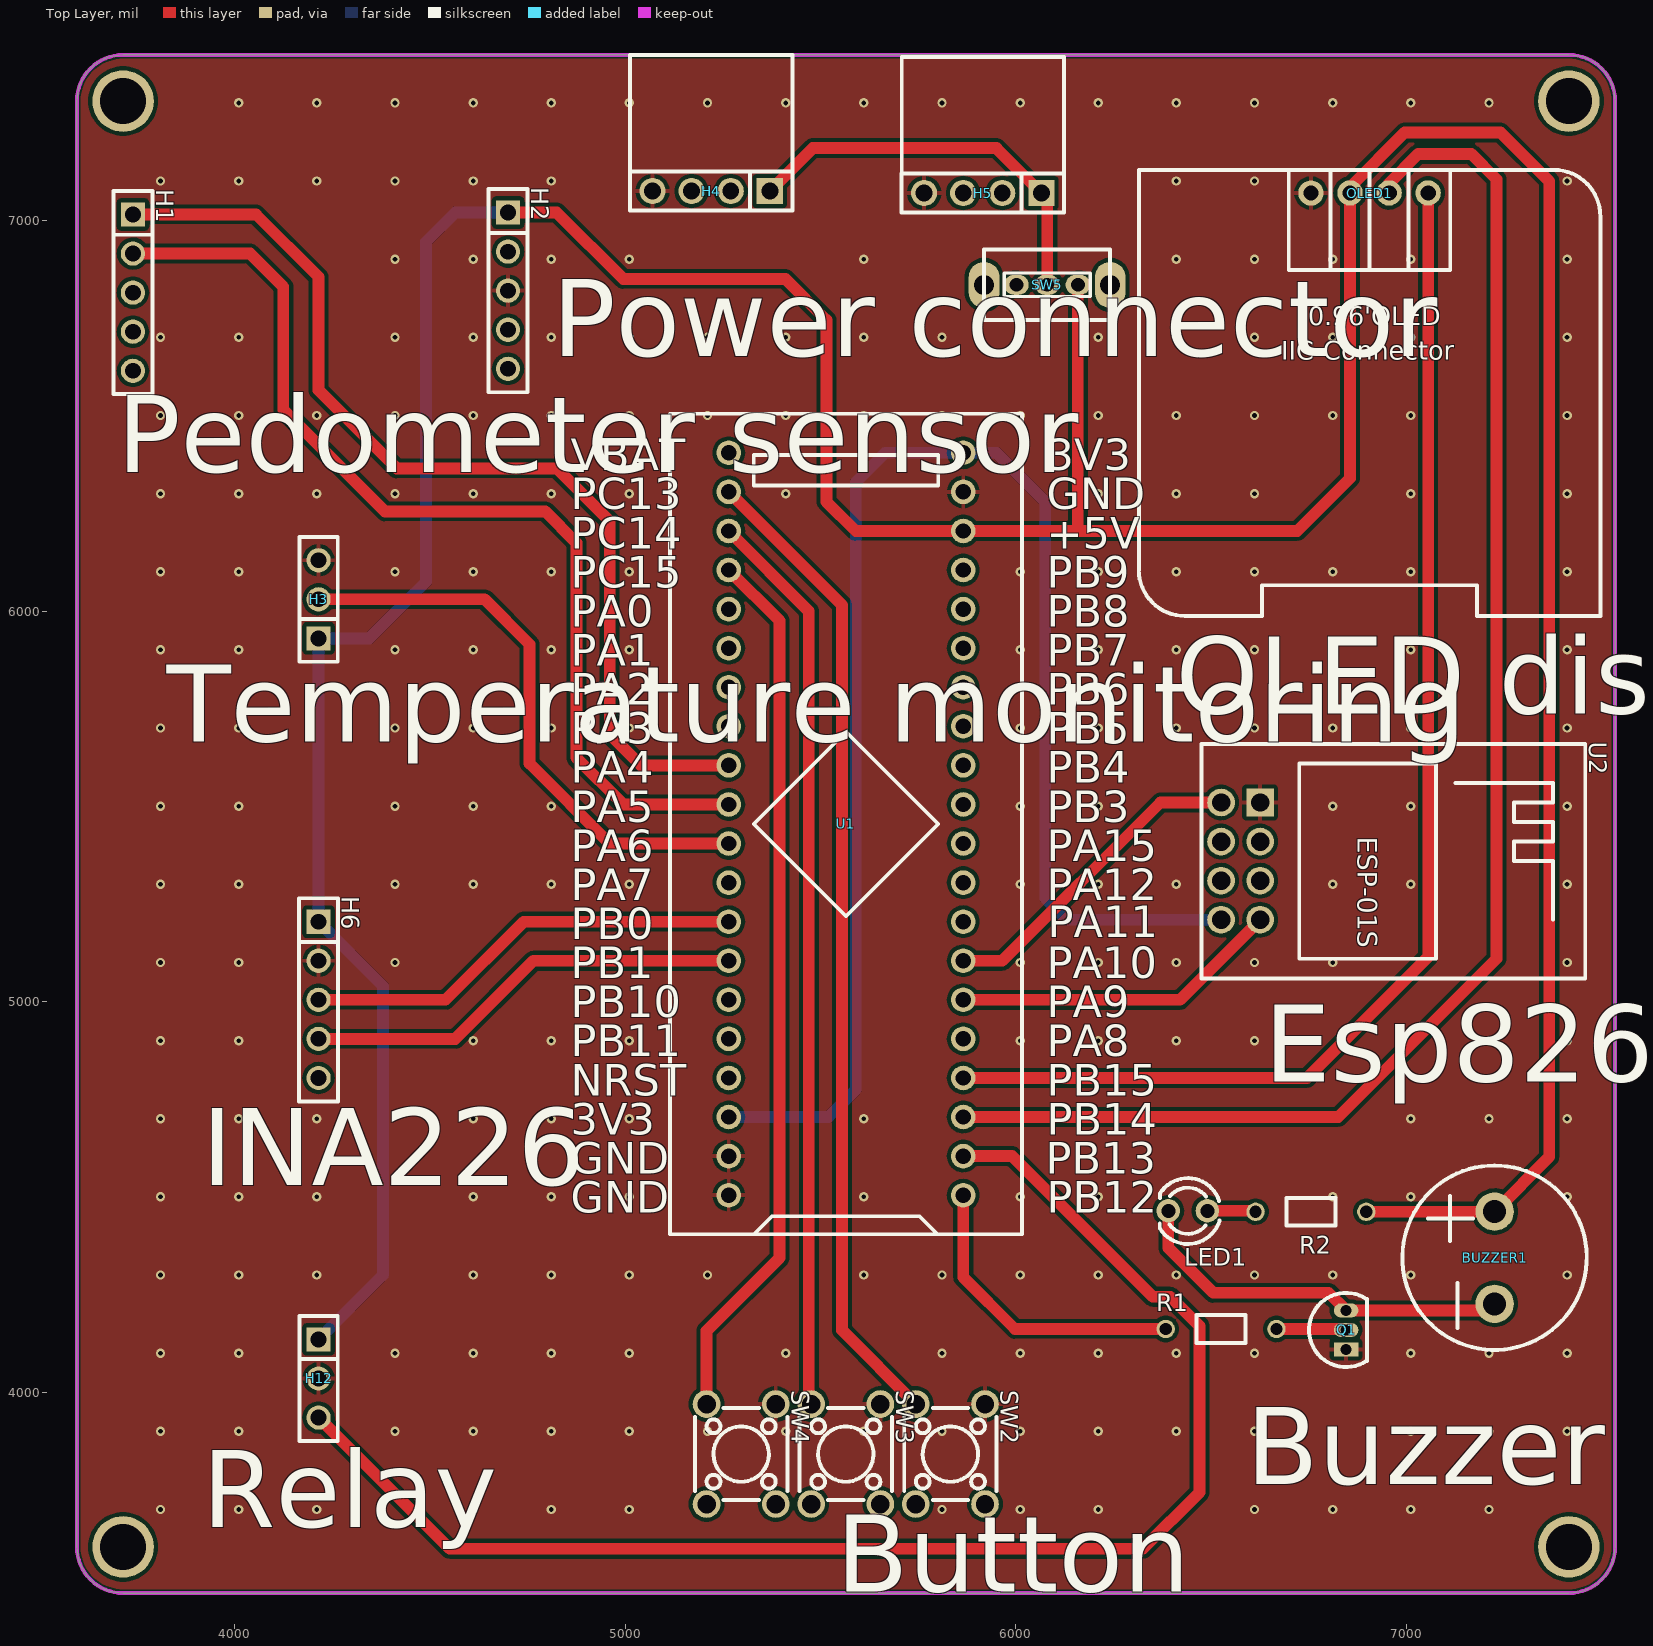
[diagram p0: Top Layer view]
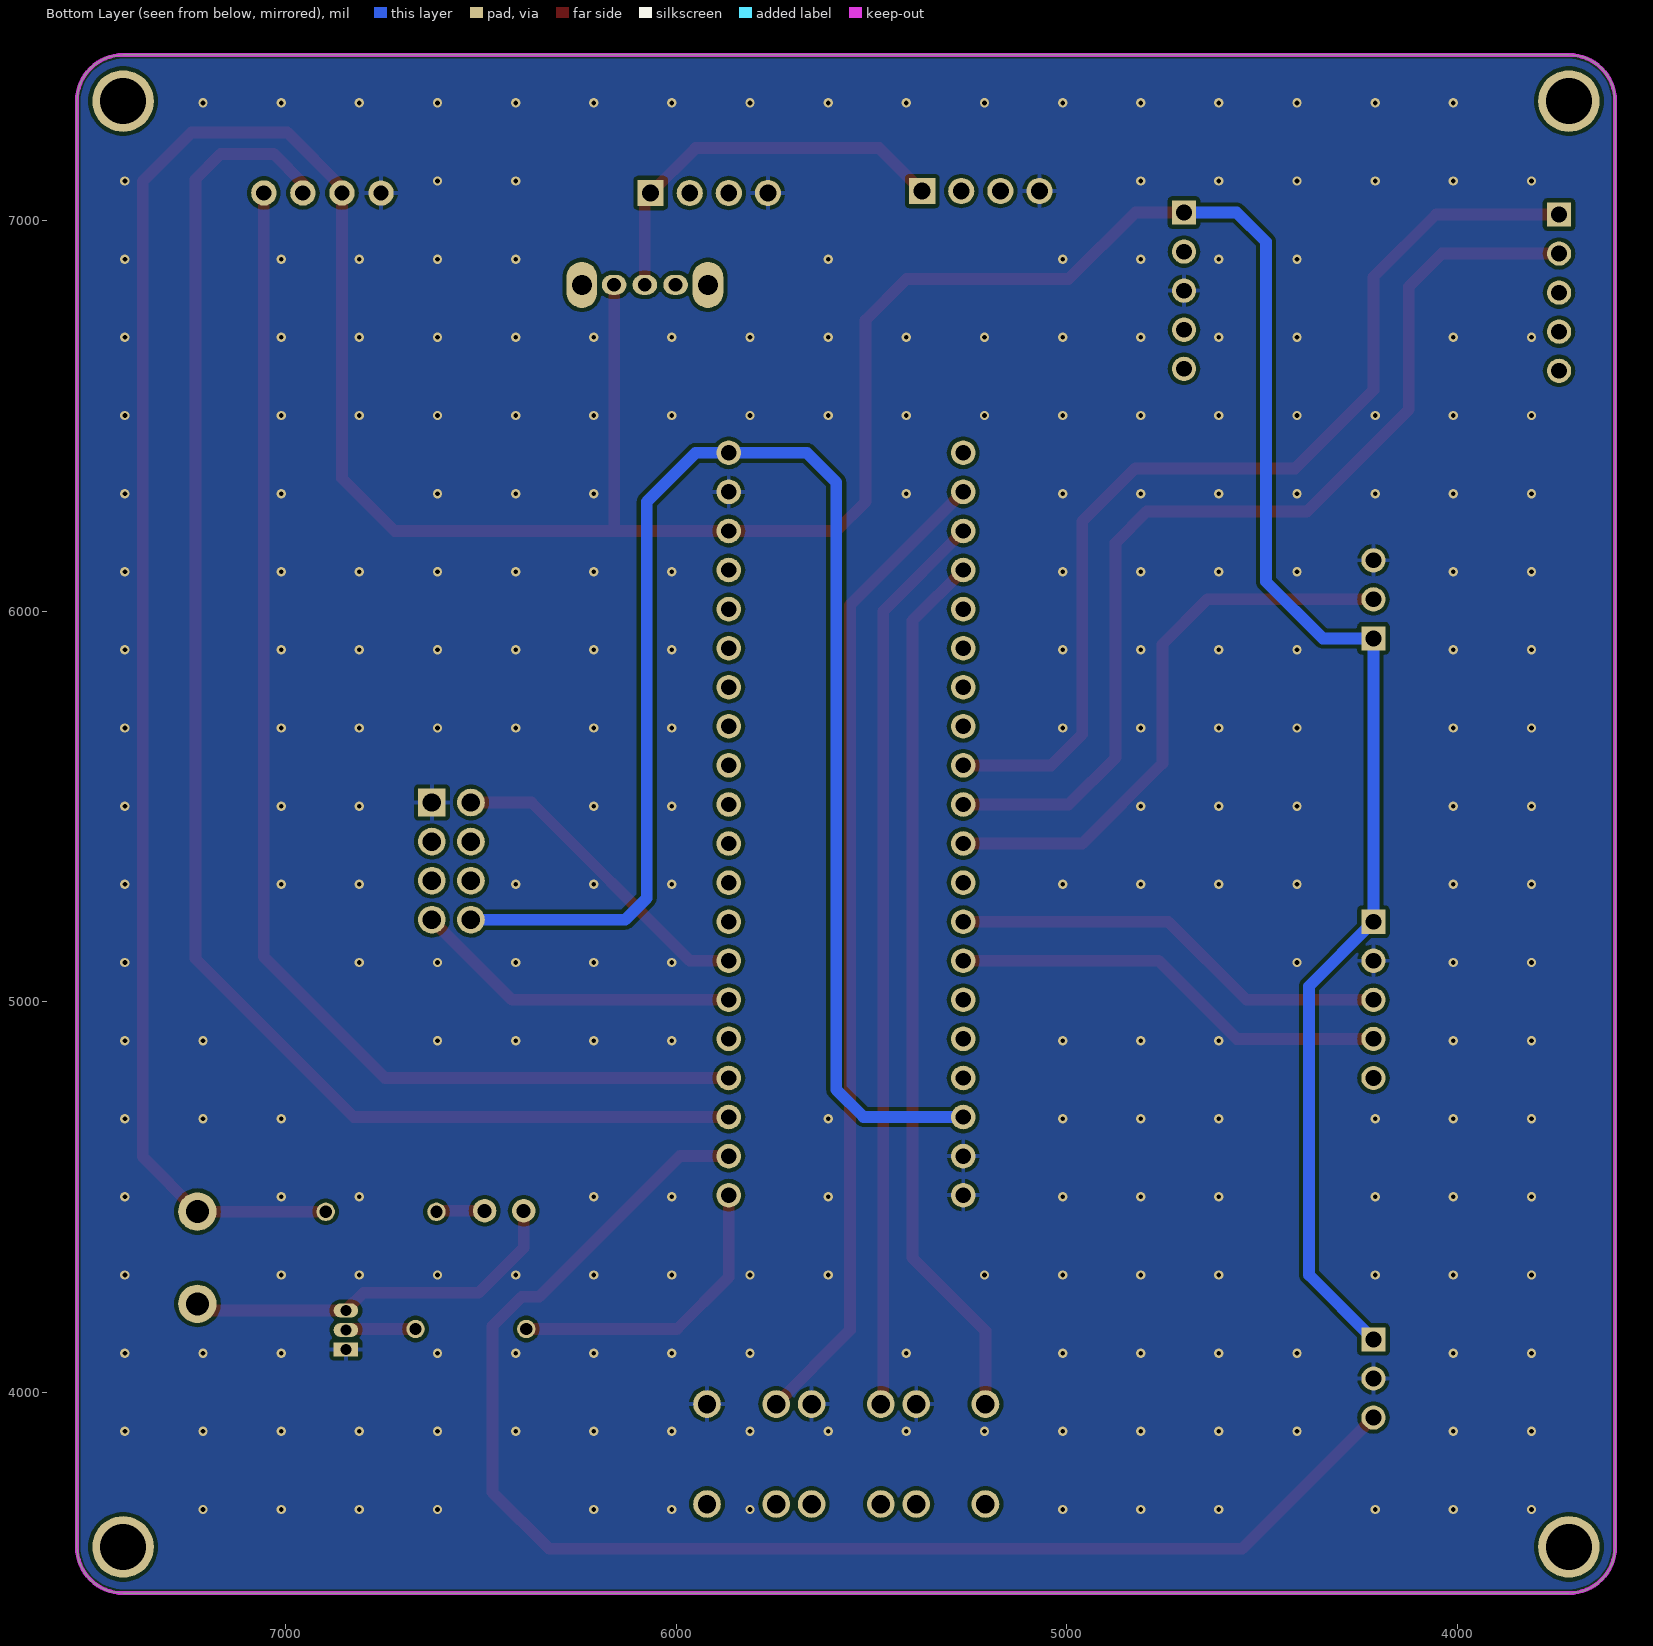
[diagram p1: Bottom Layer view, seen from below]
# Altium PCB MISC89063.pcbdoc
Units mil, origin at the board's own origin, x right, y up, seen from the top; angles counter-clockwise.
Board outline 3937.01 x 3937.01 mil, 2 copper layers (Top Layer, Bottom Layer), stack 62.206 mil thick; 19 components, 41 nets, 113 pads, 249 vias.

## Layer stack, top to bottom
Top Solder Mask Layer: solder mask 0.394, Dk 3.3
Top Layer: signal copper 1.379
Dielectric1: surface 59.449, FR4, Dk 4.5
Bottom Layer: signal copper 1.378
Bottom Solder Mask Layer: solder mask 0.394, Dk 3.3

## Board outline
3714.61,7423.5 ccw(c3714.61,7305.39) 3596.5,7305.39 3596.5,3604.61 ccw(c3714.61,3604.61) 3714.61,3486.5 7415.39,3486.5 ccw(c7415.39,3604.61) 7533.5,3604.61 7533.5,7305.39 ccw(c7415.39,7305.39) 7415.39,7423.5

## Design rules (kind name [scope] priority, off if disabled: settings)
BoardOutlineClearance copperThickness2oz_1 [All] p2 off: genericclearance=7.99 ignorepadtopadclearanceinfootprint=FALSE except(0: Arc-SplitContinuation Track-SplitContinuation SMDPad-SplitContinuation THPad-SplitContinuation Via-SplitContinuation Fill-SplitContinuation Region-SplitContinuation Poly-SplitContinuation Text-SplitContinuation Hole-SplitContinuation; 5.98: Arc-CutoutEdge Track-CutoutEdge SMDPad-CutoutEdge THPad-CutoutEdge Via-CutoutEdge Text-CutoutEdge; 6.9: Hole-OutlineEdge Hole-CutoutEdge; 10: Poly-OutlineEdge Poly-CutoutEdge; 11.81: Arc-OutlineEdge Track-OutlineEdge SMDPad-OutlineEdge THPad-OutlineEdge Via-OutlineEdge Fill-OutlineEdge Region-OutlineEdge Text-OutlineEdge Fill-CutoutEdge Region-CutoutEdge)
BoardOutlineClearance Plane_innerPlane_1 [All] p4 off: genericclearance=4.02 ignorepadtopadclearanceinfootprint=FALSE except(0: Arc-SplitContinuation Track-SplitContinuation SMDPad-SplitContinuation THPad-SplitContinuation Via-SplitContinuation Fill-SplitContinuation Region-SplitContinuation Poly-SplitContinuation Text-SplitContinuation Hole-SplitContinuation; 5.98: Arc-CutoutEdge Track-CutoutEdge SMDPad-CutoutEdge THPad-CutoutEdge Via-CutoutEdge Text-CutoutEdge; 6.9: Hole-OutlineEdge Hole-CutoutEdge; 10: Poly-OutlineEdge Poly-CutoutEdge; 11.81: Arc-OutlineEdge Track-OutlineEdge SMDPad-OutlineEdge THPad-OutlineEdge Via-OutlineEdge Fill-OutlineEdge Region-OutlineEdge Text-OutlineEdge Fill-CutoutEdge Region-CutoutEdge)
BoardOutlineClearance Copper_copperRegion_1 [All] p6 off: genericclearance=4.02 ignorepadtopadclearanceinfootprint=FALSE except(0: Arc-SplitContinuation Track-SplitContinuation SMDPad-SplitContinuation THPad-SplitContinuation Via-SplitContinuation Fill-SplitContinuation Region-SplitContinuation Poly-SplitContinuation Text-SplitContinuation Hole-SplitContinuation; 5.98: Arc-CutoutEdge Track-CutoutEdge SMDPad-CutoutEdge THPad-CutoutEdge Via-CutoutEdge Text-CutoutEdge; 6.9: Hole-OutlineEdge Hole-CutoutEdge; 10: Poly-OutlineEdge Poly-CutoutEdge; 11.81: Arc-OutlineEdge Track-OutlineEdge SMDPad-OutlineEdge THPad-OutlineEdge Via-OutlineEdge Fill-OutlineEdge Region-OutlineEdge Text-OutlineEdge Fill-CutoutEdge Region-CutoutEdge)
BoardOutlineClearance copperThickness1oz_1 [All] p8: genericclearance=4.02 ignorepadtopadclearanceinfootprint=FALSE except(0: Arc-SplitContinuation Track-SplitContinuation SMDPad-SplitContinuation THPad-SplitContinuation Via-SplitContinuation Fill-SplitContinuation Region-SplitContinuation Poly-SplitContinuation Text-SplitContinuation Hole-SplitContinuation; 5.98: Arc-CutoutEdge Track-CutoutEdge SMDPad-CutoutEdge THPad-CutoutEdge Via-CutoutEdge Text-CutoutEdge; 6.9: Hole-OutlineEdge Hole-CutoutEdge; 10: Poly-OutlineEdge Poly-CutoutEdge; 11.81: Arc-OutlineEdge Track-OutlineEdge SMDPad-OutlineEdge THPad-OutlineEdge Via-OutlineEdge Fill-OutlineEdge Region-OutlineEdge Text-OutlineEdge Fill-CutoutEdge Region-CutoutEdge)
Clearance copperThickness2oz [All] p1 off: gap=7.99 ignorepadtopadclearanceinfootprint=FALSE except(5.98: SMDPad-Track SMDPad-SMDPad THPad-Track SMDPad-THPad THPad-THPad Track-Via SMDPad-Via THPad-Via Via-Via Fill-SMDPad Region-SMDPad Fill-THPad Region-THPad Fill-Via Region-Via Fill-Fill Fill-Region Region-Region Arc-Track Arc-SMDPad Arc-THPad Arc-Via Fill-Arc Region-Arc Arc-Arc Text-Track SMDPad-Text Text-THPad Text-Via Fill-Text Region-Text Arc-Text Text-Text; 6.9: Hole-Track Hole-SMDPad Hole-THPad Hole-Via Fill-Hole Region-Hole Hole-Arc Hole-Text; 10: Poly-Track Poly-SMDPad Poly-THPad Poly-Via Poly-Fill Poly-Region Poly-Poly Poly-Arc Poly-Text Poly-Hole; 11.81: Fill-Track Region-Track)
Clearance Plane_innerPlane [All] p3 off: gap=4.02 ignorepadtopadclearanceinfootprint=FALSE except(5.98: SMDPad-Track SMDPad-SMDPad THPad-Track SMDPad-THPad THPad-THPad Track-Via SMDPad-Via THPad-Via Via-Via Fill-SMDPad Region-SMDPad Fill-THPad Region-THPad Fill-Via Region-Via Fill-Fill Fill-Region Region-Region Arc-Track Arc-SMDPad Arc-THPad Arc-Via Fill-Arc Region-Arc Arc-Arc Text-Track SMDPad-Text Text-THPad Text-Via Fill-Text Region-Text Arc-Text Text-Text; 6.9: Hole-Track Hole-SMDPad Hole-THPad Hole-Via Fill-Hole Region-Hole Hole-Arc Hole-Text; 10: Poly-Track Poly-SMDPad Poly-THPad Poly-Via Poly-Fill Poly-Region Poly-Poly Poly-Arc Poly-Text Poly-Hole; 11.81: Fill-Track Region-Track)
Clearance Copper_copperRegion [All] p5 off: gap=4.02 ignorepadtopadclearanceinfootprint=FALSE except(5.98: SMDPad-Track SMDPad-SMDPad THPad-Track SMDPad-THPad THPad-THPad Track-Via SMDPad-Via THPad-Via Via-Via Fill-SMDPad Region-SMDPad Fill-THPad Region-THPad Fill-Via Region-Via Fill-Fill Fill-Region Region-Region Arc-Track Arc-SMDPad Arc-THPad Arc-Via Fill-Arc Region-Arc Arc-Arc Text-Track SMDPad-Text Text-THPad Text-Via Fill-Text Region-Text Arc-Text Text-Text; 6.9: Hole-Track Hole-SMDPad Hole-THPad Hole-Via Fill-Hole Region-Hole Hole-Arc Hole-Text; 10: Poly-Track Poly-SMDPad Poly-THPad Poly-Via Poly-Fill Poly-Region Poly-Poly Poly-Arc Poly-Text Poly-Hole; 11.81: Fill-Track Region-Track)
Clearance copperThickness1oz [All] p7: gap=4.02 ignorepadtopadclearanceinfootprint=FALSE except(5.98: SMDPad-Track SMDPad-SMDPad THPad-Track SMDPad-THPad THPad-THPad Track-Via SMDPad-Via THPad-Via Via-Via Fill-SMDPad Region-SMDPad Fill-THPad Region-THPad Fill-Via Region-Via Fill-Fill Fill-Region Region-Region Arc-Track Arc-SMDPad Arc-THPad Arc-Via Fill-Arc Region-Arc Arc-Arc Text-Track SMDPad-Text Text-THPad Text-Via Fill-Text Region-Text Arc-Text Text-Text; 6.9: Hole-Track Hole-SMDPad Hole-THPad Hole-Via Fill-Hole Region-Hole Hole-Arc Hole-Text; 10: Poly-Track Poly-SMDPad Poly-THPad Poly-Via Poly-Fill Poly-Region Poly-Poly Poly-Arc Poly-Text Poly-Hole; 11.81: Fill-Track Region-Track)
DiffPairsRouting differentialPair [All] p1: maxlimit=6 minlimit=6 mostfreqgap=6 toplayer_minwidth=5 toplayer_prefwidth=10 toplayer_maxwidth=100 toplayer_mingap=6 toplayer_prefgap=6 toplayer_maxgap=6 bottomlayer_minwidth=5 bottomlayer_prefwidth=10 bottomlayer_maxwidth=100 bottomlayer_mingap=6 bottomlayer_prefgap=6 bottomlayer_maxgap=6 maxuncoupledlength=10
HoleToHoleClearance otherClearance [All] p1: gap=11.81 allowstackedmicrovias=TRUE
Length netLength [All] p1: minlimit=0 maxlimit=0
PasteMaskExpansion pasteMaskExpansion [All] p1: expansion=0
PlaneConnect innerPlane [All] p1: planeconnectstyle=Relief reliefexpansion=20 reliefentries=4 reliefconductorwidth=10 reliefairgap=10
PolygonConnect copperRegion [All] p1: connectstyle=Relief reliefconductorwidth=10 reliefentries=4 polygonreliefangle="90 Angle" airgapwidth=10 via.connectstyle=Relief via.reliefconductorwidth=10 via.reliefentries=4 via.polygonreliefangle="90 Angle" via.airgapwidth=10
RoutingVias viaSize [All] p1: holewidth=12.01 width=24.02 viastyle="Through Hole" minholewidth=11.81 minwidth=19.68 maxholewidth=248.03 maxwidth=393.7
SolderMaskExpansion solderMaskExpansion [IsVia] p1: expansion=-1000 istentingtop=TRUE
SolderMaskExpansion solderMaskExpansion [All] p2: expansion=2 istentingtop=FALSE
Width copperThickness2oz_2 [All] p1 off: maxlimit=100 minlimit=8 preferedwidth=10
Width copperThickness1oz_2 [All] p2: maxlimit=100 minlimit=5 preferedwidth=10

## Components (designator, comment, footprint, x,y, rotation, side; value= is the part's Value field where it differs from the comment)
BUZZER1 "buzzer" BUZ-TH_BD12.0-P6.00-D0.9-RD 7225,4345 r90 top
H1 "" HDR-TH_5P-P2.54-V-F 3740,6815 r270 top
H2 "" HDR-TH_5P-P2.54-V-F 4700,6820 r270 top
H3 "" HDR-TH_3P-P2.54-V-F 4215,6030 r90 top
H4 "" HDR-TH_4P-P2.54-V-F 5220,7075 r180 top
H5 "" HDR-TH_4P-P2.54-V-F 5915,7070 r180 top
H6 "" HDR-TH_5P-P2.54-V-F 4215,5005 r270 top
H12 "" HDR-TH_3P-P2.54-V-F 4215,4035.79 r270 top
LED1 "" LED_TH-3mm 6440,4465 r180 top
OLED1 "" 0.96OLED_4P 6905,7070 r0 top
Q1 "" S8050_TO_92 6845,4160 r90 top
R1 "100Ω" Res_1/8W 6525,4160 r0 top
R2 "1kΩ" Res_1/8W 6755,4460 r0 top
SW2 "" SW-TH_4P-L6.0-W6.0-P4.50-LS6.5 5832.14,3842.47 r270 top
SW3 "" SW-TH_4P-L6.0-W6.0-P4.50-LS6.5 5564.43,3842.47 r270 top
SW4 "" SW-TH_4P-L6.0-W6.0-P4.50-LS6.5 5296.72,3842.47 r270 top
SW5 "" 拨动开关 6085,6835 r180 top
U1 "STM32F103C8T6-Card" CONN-TH_L53.3-W22.9_STM32F103C8T6-CARD 5565,5455 r90 top
U2 "ESP-01S" WIFIM-TH_ESP-01S 6575,5360 r270 top

## Footprints (in the part's own frame and the unit in brackets; to place one, negate y for a bottom-side part, rotate by r counter-clockwise, add the part's x,y. Pads: shape width x height; smd on the part's side, far side on the other; paste and mask are expansions set on the pad)
0.96OLED_4P [mm]
  round 1.65 hole 1 copper offset 0,0: 1(-3.81,-0.001) 2(-1.27,0.002) 3(1.27,0.002) 4(3.81,0.002)
  silkscreen extent -15,-27.5 15,1.5
BUZ-TH_BD12.0-P6.00-D0.9-RD [mm]
  round 2.5 hole 1.5 paste+0 mask+0.05: 1(-3,0) 2(3,0)
  silkscreen extent -5.99,-5.99 5.99,5.99
CONN-TH_L53.3-W22.9_STM32F103C8T6-CARD [mm]
  round 1.6 hole 1: 1(-24.13,-7.62) 2(-21.59,-7.62) 3(-19.05,-7.62) 4(-16.51,-7.62) 5(-13.97,-7.62) 6(-11.43,-7.62) 7(-8.89,-7.62) 8(-6.35,-7.62) 9(-3.81,-7.62) 10(-1.27,-7.62) 11(1.27,-7.62) 12(3.81,-7.62) 13(6.35,-7.62) 14(8.89,-7.62) 15(11.43,-7.62) 16(13.97,-7.62) 17(16.51,-7.62) 18(19.05,-7.62) 19(21.59,-7.62) 20(24.13,-7.62) 21(24.13,7.62) 22(21.59,7.62) 23(19.05,7.62) 24(16.51,7.62) 25(13.97,7.62) 26(11.43,7.62) 27(8.89,7.62) 28(6.35,7.62) 29(3.81,7.62) 30(1.27,7.62) 31(-1.27,7.62) 32(-3.81,7.62) 33(-6.35,7.62) 34(-8.89,7.62) 35(-11.43,7.62) 36(-13.97,7.62) 37(-16.51,7.62) 38(-19.05,7.62) 39(-21.59,7.62) 40(-24.13,7.62)
  silkscreen extent -26.67,-11.43 26.67,11.43
HDR-TH_3P-P2.54-V-F [mil]
  rect 62x62 hole 40.16: 1(-100,0)
  round 62 hole 40.16: 2(0,0) 3(100,0)
  silkscreen extent -160,-49 160,49
HDR-TH_4P-P2.54-V-F [mm]
  rect 1.7x1.7 hole 1.1: 1(-3.81,0)
  round 1.7 hole 1.1: 2(-1.27,0) 3(1.27,0) 4(3.81,0)
  silkscreen extent -5.29,-1.27 5.29,1.27
HDR-TH_5P-P2.54-V-F [mil]
  rect 62x62 hole 40.16: 1(-200,0)
  round 62 hole 40.16: 2(-100,0) 3(0,0) 4(100,0) 5(200,0)
  silkscreen extent -260,-50 260,50
LED_TH-3mm [mil]
  round 60 hole 36 paste+0 mask+2: 1(-50,0) 2(50,0)
  silkscreen extent -81,-84 72,85
Res_1/8W [mil]
  round 47.2 hole 31.5 paste+0 mask+2: 1(-141.7,2.48) 2(141.7,2.48)
  silkscreen extent -63,-33 63,38
S8050_TO_92 [mil]
  rect 35.4x63 hole 27.6 paste+0 mask+2: 1(-50,0)
  oval 35.4x63 hole 27.6 paste+0 mask+2: 2(0,0) 3(50,0)
  silkscreen extent -95,-53 95,95
SW-TH_4P-L6.0-W6.0-P4.50-LS6.5 [mm]
  round 1.8 hole 1.2: 1(-3.25,2.25) 2(3.25,2.25) 3(-3.25,-2.25) 4(3.25,-2.25)
  silkscreen extent -3,-3 3,3
WIFIM-TH_ESP-01S [mm]
  rect 1.8x1.8 hole 1.2: 1(-3.81,1.27)
  round 1.8 hole 1.2: 2(-1.27,1.27) 3(1.27,1.27) 4(3.81,1.27) 5(3.81,-1.27) 6(1.27,-1.27) 7(-1.27,-1.27) 8(-3.81,-1.27)
  silkscreen extent -7.62,-2.54 7.62,22.4
拨动开关 [mil]
  oval 63x51.2 hole 35.4 paste+0 mask+2: 1(-73.4,0) 2(5,0) 3(84,0)
  oval 78.7x118.1 hole 51.2 paste+0 mask+2: 4(166.7,0) 5(-156.1,0)
  silkscreen extent -156,-90 167,90

## Free pads (board coordinates)
  round 157.48 hole 118.11: 1(3714.61,7305.39) 1(3714.61,3604.61) 1(7415.39,7305.39) 1(7415.39,3604.61)

## Via types
v1: diameter 24.02, hole 12, Top Layer to Bottom Layer, 249 vias

## Nets (pads, with @x,y where several pads share a name; then routed paths per layer and width w, separated by ;. In a path a pad name is that pad's centre, name@x,y a point inside that pad or via, vN(x,y) a via of type N, cw(c..) or ccw(c..) an arc to the next point about the centre after c; other vN are vias at no path point)
3.3V: U1.20 U1.38 U2.5 | length 3964.6
  Bottom Layer w30: U1.38 5520,4705 5590,4775 5590,6330 5665,6405 U1.20 5950,6405 6075,6280 6075,5265 6130,5210 U2.5
$1N17118: H4.1 H5.1 SW5.2 | length 1029.4
  Top Layer w30: H4.1 5480,7185 5950,7185 H5.1 6080,7055 SW5.2
$1N17139: BUZZER1.1 LED1.2 Q1.3 | length 1003.3
  Top Layer w30: LED1.2 6390,4370 6505,4255 6800,4255 Q1.3 7208.11,4210 BUZZER1.1
$1N17142: Q1.2 R1.2 | length 179.3
  Top Layer w30: R1.2 6842.52,4162.48 Q1.2
$1N17145: LED1.1 R2.1 | length 124.3
  Top Layer w30: LED1.1 6610.78,4465 R2.1
GND: H2.3 H3.3 H4.4 H5.4 H6.2 H12.2 OLED1.1 Q1.1 SW2.1 SW3.1 SW4.1 U1.19 U1.39 U1.40 U2.1
  other v1: 3810.6,3700.6 4010.6,3700.6 4210.6,3700.6 4610.6,3700.6 4810.6,3700.6 5010.6,3700.6 5810.6,3700.6 6010.6,3700.6 6210.6,3700.6 6610.6,3700.6 6810.6,3700.6 7010.6,3700.6 7210.6,3700.6 3810.6,3900.6 4010.6,3900.6 4410.6,3900.6 4610.6,3900.6 4810.6,3900.6 5010.6,3900.6 5210.6,3900.6 5410.6,3900.6 5610.6,3900.6 5810.6,3900.6 6010.6,3900.6 6210.6,3900.6 6410.6,3900.6 6610.6,3900.6 6810.6,3900.6 7010.6,3900.6 7210.6,3900.6 7410.6,3900.6 3810.6,4100.6 4010.6,4100.6 4410.6,4100.6 4610.6,4100.6 4810.6,4100.6 5010.6,4100.6 5410.6,4100.6 5810.6,4100.6 6010.6,4100.6 6210.6,4100.6 6410.6,4100.6 6610.6,4100.6 7010.6,4100.6 7210.6,4100.6 7410.6,4100.6 3810.6,4300.6 4010.6,4300.6 4210.6,4300.6 4610.6,4300.6 4810.6,4300.6 5010.6,4300.6 5210.6,4300.6 5610.6,4300.6 5810.6,4300.6 6010.6,4300.6 6210.6,4300.6 6410.6,4300.6 6610.6,4300.6 6810.6,4300.6 7010.6,4300.6 7410.6,4300.6 3810.6,4500.6 4010.6,4500.6 4210.6,4500.6 4610.6,4500.6 4810.6,4500.6 5010.6,4500.6 5610.6,4500.6 6010.6,4500.6 6210.6,4500.6 6810.6,4500.6 7010.6,4500.6 7410.6,4500.6 3810.6,4700.6 4010.6,4700.6 4210.6,4700.6 4610.6,4700.6 4810.6,4700.6 5010.6,4700.6 5610.6,4700.6 7010.6,4700.6 7210.6,4700.6 7410.6,4700.6 3810.6,4900.6 4010.6,4900.6 4610.6,4900.6 4810.6,4900.6 5010.6,4900.6 6010.6,4900.6 6210.6,4900.6 6410.6,4900.6 6610.6,4900.6 7210.6,4900.6 7410.6,4900.6 3810.6,5100.6 4010.6,5100.6 4410.6,5100.6 6010.6,5100.6 6210.6,5100.6 6410.6,5100.6 6610.6,5100.6 6810.6,5100.6 7410.6,5100.6 3810.6,5300.6 4010.6,5300.6 4410.6,5300.6 4610.6,5300.6 4810.6,5300.6 5010.6,5300.6 6010.6,5300.6 6210.6,5300.6 6410.6,5300.6 6810.6,5300.6 7010.6,5300.6 7410.6,5300.6 3810.6,5500.6 4010.6,5500.6 4410.6,5500.6 4610.6,5500.6 4810.6,5500.6 6010.6,5500.6 6210.6,5500.6 6810.6,5500.6 7010.6,5500.6 7410.6,5500.6 3810.6,5700.6 4010.6,5700.6 4410.6,5700.6 4610.6,5700.6 4810.6,5700.6 5010.6,5700.6 6010.6,5700.6 6210.6,5700.6 6410.6,5700.6 6610.6,5700.6 6810.6,5700.6 7010.6,5700.6 7410.6,5700.6 3810.6,5900.6 4010.6,5900.6 4410.6,5900.6 4610.6,5900.6 4810.6,5900.6 5010.6,5900.6 6010.6,5900.6 6210.6,5900.6 6410.6,5900.6 6610.6,5900.6 6810.6,5900.6 7010.6,5900.6 7410.6,5900.6 3810.6,6100.6 4010.6,6100.6 4410.6,6100.6 4610.6,6100.6 4810.6,6100.6 5010.6,6100.6 6010.6,6100.6 6210.6,6100.6 6410.6,6100.6 6610.6,6100.6 6810.6,6100.6 7010.6,6100.6 7410.6,6100.6 3810.6,6300.6 4010.6,6300.6 4210.6,6300.6 4410.6,6300.6 4610.6,6300.6 4810.6,6300.6 5010.6,6300.6 5410.6,6300.6 6210.6,6300.6 6410.6,6300.6 6610.6,6300.6 7010.6,6300.6 7410.6,6300.6 3810.6,6500.6 4010.6,6500.6 4210.6,6500.6 4410.6,6500.6 4610.6,6500.6 4810.6,6500.6 5010.6,6500.6 5210.6,6500.6 5410.6,6500.6 5610.6,6500.6 5810.6,6500.6 6010.6,6500.6 6210.6,6500.6 6410.6,6500.6 6610.6,6500.6 6810.6,6500.6 7010.6,6500.6 7410.6,6500.6 3810.6,6700.6 4010.6,6700.6 4410.6,6700.6 4610.6,6700.6 4810.6,6700.6 5010.6,6700.6 5210.6,6700.6 5410.6,6700.6 5610.6,6700.6 5810.6,6700.6 6010.6,6700.6 6210.6,6700.6 6410.6,6700.6 6610.6,6700.6 6810.6,6700.6 7010.6,6700.6 7410.6,6700.6 4410.6,6900.6 4610.6,6900.6 4810.6,6900.6 5010.6,6900.6 5610.6,6900.6 6410.6,6900.6 6610.6,6900.6 6810.6,6900.6 7010.6,6900.6 7410.6,6900.6 3810.6,7100.6 4010.6,7100.6 4210.6,7100.6 4410.6,7100.6 4610.6,7100.6 4810.6,7100.6 6410.6,7100.6 6610.6,7100.6 7410.6,7100.6 4010.6,7300.6 4210.6,7300.6 4410.6,7300.6 4610.6,7300.6 4810.6,7300.6 5010.6,7300.6 5210.6,7300.6 5410.6,7300.6 5610.6,7300.6 5810.6,7300.6 6010.6,7300.6 6210.6,7300.6 6410.6,7300.6 6610.6,7300.6 6810.6,7300.6 7010.6,7300.6 7210.6,7300.6
NRST: U1.37
PA0: U1.25
PA1: U1.26
PA2: U1.27
PA3: U1.28
PA4: H1.1 U1.29 | length 2598.2
  Top Layer w30: H1.1 4055,7015 4215,6855 4215,6565 4415,6365 4825,6365 4960,6230 4960,5685 5040,5605 U1.29
PA5: H1.2 U1.30 | length 2615.7
  Top Layer w30: H1.2 4040,6915 4125,6830 4125,6515 4385,6255 4795,6255 4875,6175 4875,5625 4995,5505 U1.30
PA6: H3.2 U1.31 | length 1487.5
  Top Layer w30: H3.2 4640,6030 4755,5915 4755,5610 4960,5405 U1.31
PA7: U1.32
PA8: U1.5
PA9: U1.6 U2.4 | length 844.9
  Top Layer w30: U1.6 6420,5005 U2.4
PA10: U1.7 U2.8 | length 827.8
  Top Layer w30: U1.7 5965,5105 6370,5510 U2.8
PA11: U1.8
PA12: U1.9
PA15: U1.10
PB0: H6.3 U1.33 | length 1132.8
  Top Layer w30: H6.3 4540,5005 4740,5205 U1.33
PB1: H6.4 U1.34 | length 1132.8
  Top Layer w30: H6.4 4565,4905 4765,5105 U1.34
PB3: U1.11
PB4: U1.12
PB5: U1.13
PB6: U1.14
PB7: U1.15
PB8: U1.16
PB9: U1.17
PB10: U1.35
PB11: U1.36
PB12: R1.1 U1.1 | length 783.2
  Top Layer w30: U1.1 5865,4295 5997.52,4162.48 R1.1
PB13: H12.3 U1.2 | length 3664.3
  Top Layer w30: H12.3 4550.79,3600 6325,3600 6470,3745 6470,4170 6395,4245 6350,4245 5990,4605 U1.2
PB14: OLED1.3 U1.3 | length 3885.7
  Top Layer w30: U1.3 6825,4705 7230,5110 7230,7105 7165,7170 7030,7170 6955,7095 OLED1.3@6955,7070.05
PB15: OLED1.4 U1.4 | length 3273.5
  Top Layer w30: U1.4 6745,4805 7055,5115 OLED1.4@7055,7070.05
PC13: SW2.3 U1.22 | length 2532.8
  Top Layer w30: U1.22 5555,6015 5555,4158.98 SW2.3
PC14: SW3.3 U1.23 | length 2321.9
  Top Layer w30: U1.23 5470,6000 5470,3976.27 SW3.3
PC15: SW4.3 U1.24 | length 2265.8
  Top Layer w30: SW4.3 5208.14,4158.14 5395,4345 5395,5975 U1.24
VBAT: U1.21
VCC: BUZZER1.2 H2.1 H3.1 H6.1 H12.1 OLED1.2 R2.2 SW5.1 U1.18 | length 11216.8
  Top Layer w30: H2.1 4825,7020 4995,6850 5410,6850 5515,6745 5515,6280 5590,6205 U1.18 6156.73,6205 ; SW5.1 6158.4,6206.67 6156.73,6205 ; R2.2 7224.37,4462.48 BUZZER1.2 7365,4603.11 7365,7100 7240,7225 6995,7225 6855,7085 6855,7070.05 6855,6340 6720,6205 6156.73,6205
  Bottom Layer w30: H12.1 4380,4300.79 4380,5040 H6.1 H3.1 4345,5930 4490,6075 4490,6945 4565,7020 H2.1
pads on no net: H1.3 H1.4 H1.5 H2.2 H2.4 H2.5 H4.2 H4.3 H5.2 H5.3 H6.5 SW2.2 SW2.4 SW3.2 SW3.4 SW4.2 SW4.4 SW5.3 SW5.4 SW5.5 U2.2 U2.3 U2.6 U2.7

## Polygon pours and split planes (outlines as drawn)
GND on Bottom Layer (solid, remove dead copper, pour order 2): 3525,7545 3525,3380 7700,3380 7700,7545
GND on Top Layer (solid, remove dead copper, pour order 2): 3000,7715 3000,3300 7930,3300 7930,7715
GND on Bottom Layer (solid, remove dead copper, pour order 4): 3160,7725 3160,3000 7965,3000 7965,7725

## Keep-outs
Board Outline Layer:
  the board outline again, w10

## Silkscreen, mask and mechanical layers (free items; w line width, h text height)
Top Silkscreen Layer:
  lines w10: 5012.67,7025 5012.67,7423.5 5428.27,7423.5 5428.27,7025 5012.67,7025 ; 5707.67,7020 5707.67,7418.5 6123.27,7418.5 6123.27,7020 5707.67,7020
  text "Power connector" at 4812.87,6651.57 h196.85
  text "VBAT" at 4860.95,6360 h80
  text "3V3" at 6079.16,6360 h80
  text "Pedometer sensor" at 3700,6355 h196.85
  text "PC13" at 4860.95,6260 h80
  text "GND" at 6079.16,6260 h80
  text "PC14" at 4860.95,6160 h80
  text "+5V" at 6079.16,6160 h80
  text "PC15" at 4860.95,6060 h80
  text "PB9" at 6079.16,6060 h80
  text "PA0" at 4860.95,5960 h80
  text "PB8" at 6079.16,5960 h80
  text "PA1" at 4860.95,5860 h80
  text "PB7" at 6079.16,5860 h80
  text "PA2" at 4860.95,5760 h80
  text "PB6" at 6079.16,5760 h80
  text "OLED display" at 6408.66,5736.57 h196.85
  text "Temperature monitoring" at 3826.97,5665 h196.85
  text "PA3" at 4860.95,5660 h80
  text "PB5" at 6079.16,5660 h80
  text "PA4" at 4860.95,5560 h80
  text "PB4" at 6079.16,5560 h80
  text "PA5" at 4860.95,5460 h80
  text "PB3" at 6079.16,5460 h80
  text "PA6" at 4860.95,5360 h80
  text "PA15" at 6079.16,5360 h80
  text "PA7" at 4860.95,5260 h80
  text "PA12" at 6079.16,5260 h80
  text "PA11" at 6080.95,5165 h80
  text "PB0" at 4860.95,5160 h80
  text "PB1" at 4860.95,5060 h80
  text "PA10" at 6079.16,5060 h80
  text "PB10" at 4860.95,4960 h80
  text "PA9" at 6079.16,4960 h80
  text "PB11" at 4860.95,4860 h80
  text "PA8" at 6079.16,4860 h80
  text "Esp8266" at 6635,4795 h196.85
  text "NRST" at 4860.95,4760 h80
  text "PB15" at 6079.16,4760 h80
  text "3V3" at 4860.95,4660 h80
  text "PB14" at 6079.16,4660 h80
  text "GND" at 4860.95,4560 h80
  text "PB13" at 6075.95,4560 h80
  text "INA226" at 3916.44,4530 h196.85
  text "GND" at 4860.95,4460 h80
  text "PB12" at 6079.16,4460 h80
  text "Buzzer" at 6590,3765 h196.85
  text "Relay" at 3917.79,3655 h196.85
  text "Button" at 5540,3490 h196.85